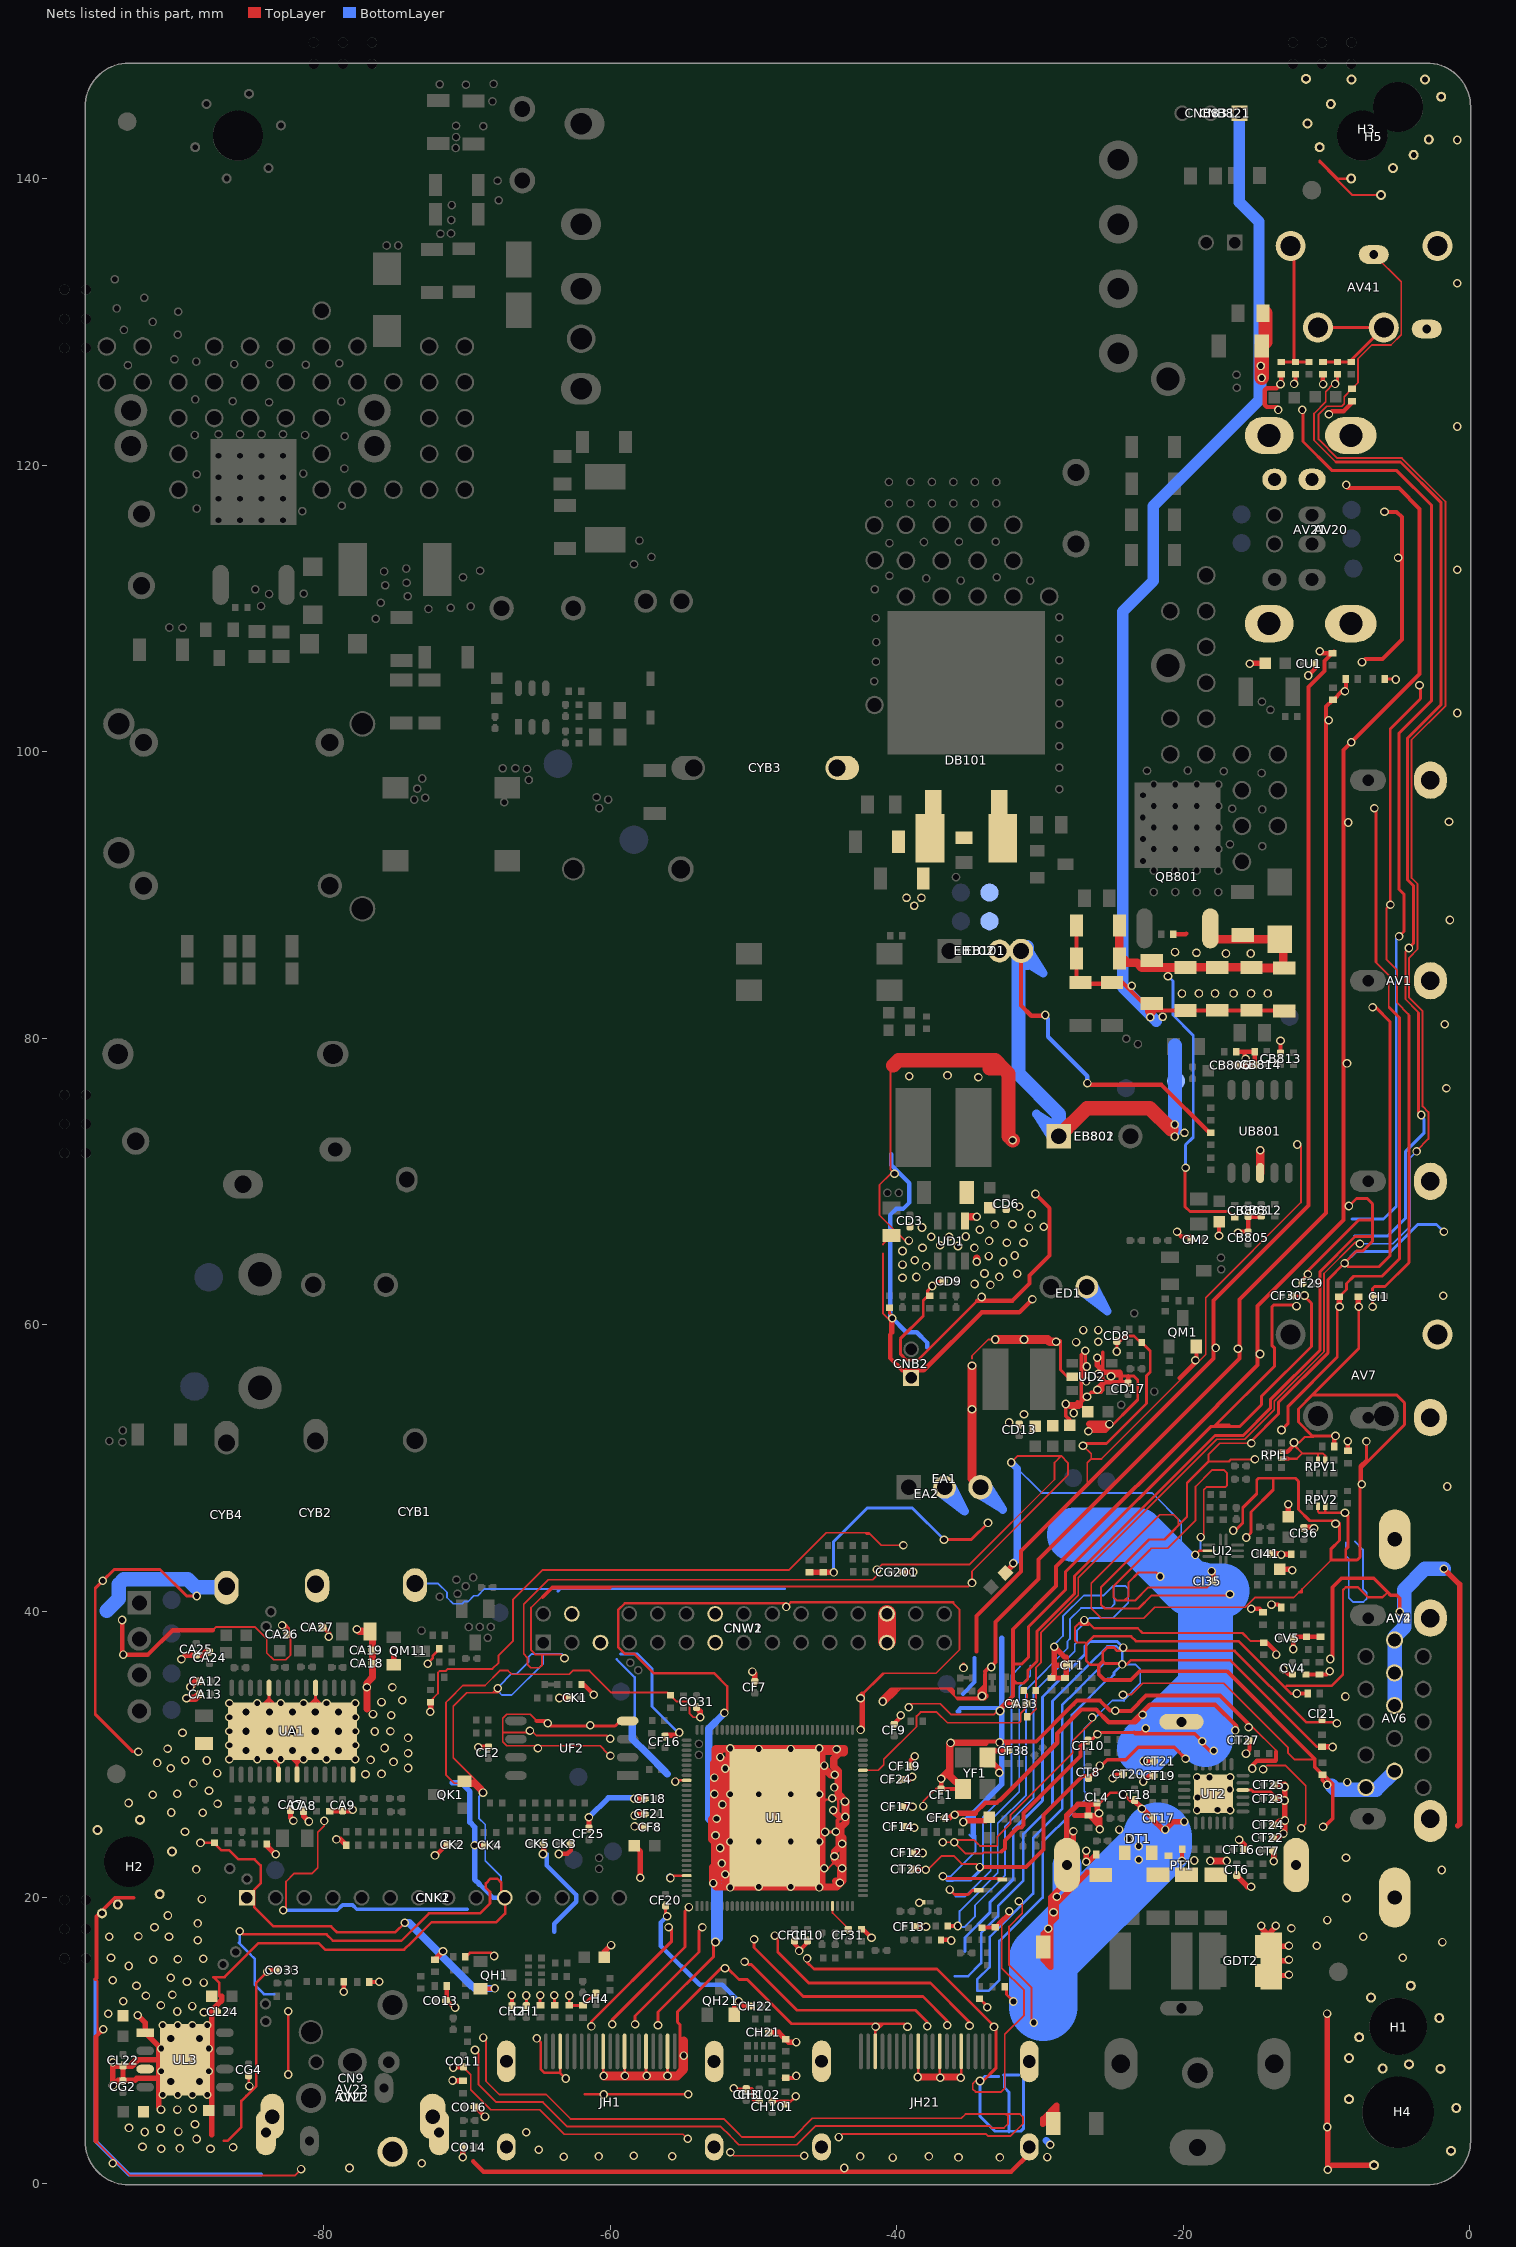
[diagram p0: the nets of this part, all layers, seen from the top]
# Altium PCB MISC86372.PcbDoc (part 8 of 16)
Units mm, origin at the board's own origin, x right, y up, seen from the top; angles counter-clockwise.
Board outline 96.73 x 148.13 mm, 2 copper layers (TopLayer, BottomLayer), stack 1.571 mm thick; 578 components, 318 nets, 2702 pads, 836 vias.

## Via types
v1: diameter 0.6, hole 0.4, TopLayer to BottomLayer, tented both sides, 816 vias
v2: diameter 0.7, hole 0.5, TopLayer to BottomLayer, tented both sides, 15 vias
v3: diameter 0.8, hole 0.5, TopLayer to BottomLayer, tented both sides, 5 vias

## Nets (pads, with @x,y where several pads share a name; then routed paths per layer and width w, separated by ;. In a path a pad name is that pad's centre, name@x,y a point inside that pad or via, vN(x,y) a via of type N, cw(c..) or ccw(c..) an arc to the next point about the centre after c; other vN are vias at no path point) (continued)
EPH_DET_IN: AV41.6 DA33.K RA35.1 RA36.2 | length 129.3
  TopLayer w0.127: RA35.1@-30.792,32.639 -30.284,33.148 RA36.2@-30.284,34.442 -30.284,36.042 -29.939,36.386 -29.939,38.482 -27.33,41.09 -27.33,42.335 -17.671,51.994 -15.703,51.994 -13.652,54.044 -13.652,54.636 ; -13.65,54.635 -10.173,58.112 -10.173,63.563 -7.991,65.746 -7.773,65.746 v1(-7.666,65.638) ; AV41.6@-6.7,134.7 -4.785,132.785 -4.785,129.097 -5.497,128.385 -6.838,128.385 -7.798,127.425 -7.798,125.751 DA33.K@-8.23,125.319 -8.766,124.783 -8.766,124.286 -8.939,124.112 -9.993,124.112 -10.554,123.551 -10.554,121.793 -9.245,120.485 -4.73,120.485 -1.702,117.456 -1.702,103.175 -4.065,100.812 -4.065,91.183 -3.645,90.763 -3.645,86.195 -4.229,85.611 -4.229,82.809 -3.289,81.869 -3.289,75.23 -2.888,74.828 -2.888,72.957 -3.708,72.136 v1(-3.708,72.085)
  BottomLayer w0.127: v1(-7.666,65.638) -5.38,65.638 -4.178,66.84 -4.178,71.615 v1(-3.708,72.085)
EPH_DET_IN_IC: CA33.2@-30.898,33.528 CA33.2@-31.073,33.528 RA36.1 U1.58 | length 16
  TopLayer w0.127: U1.58@-42.363,28.881 -41.3,28.881 -40.907,29.273 -40.907,29.646 -38.617,31.936 -38.617,32.663 -38.337,32.943 -37.204,32.943 -36.459,32.199 -31.45,32.199 -31.344,32.305 -31.344,32.872 -31.073,33.143 CA33.2@-31.073,33.528 ; RA36.1@-31.134,34.442 -30.898,34.206 CA33.2@-30.898,33.528
EPH_LOUT: AV41.4 AV41.5 DA31.K RA31.2 RA34.2 | length 9.8
  TopLayer w0.203: AV41.5@-10.6,129.6 -6.512,129.6 AV41.4@-6.256,129.344 ; DA31.K@-10.251,127.196 RA34.2@-8.27,127.196 -8.27,127.33 AV41.4@-6.256,129.344 ; AV41.4@-6,129.6 AV41.4@-6.256,129.344
EPH_ROUT: AV41.3 DA32.K RA32.2 RA33.2 | length 10.1
  TopLayer w0.203: DA32.K@-13.157,127.196 RA33.2@-11.227,127.196 ; AV41.3@-12.5,135.3 -12.268,135.068 RA32.2@-12.268,127.222
FB: CB129.2 pad.VIA5@-15.291,85.903 pad.VIA5@-17.018,85.903 pad.VIA5@-19.075,85.954 pad.VIA5@-20.574,86.004 QB801.S RB806.1 RB808.2 RB818.1 RB819.1 RB820.1 RB821.1 RB822.1 RB823.1 RB824.1 ZDB801.A | length 45.1
  TopLayer w0.2: v1@-19.866,70.942 -19.866,68.224 -19.533,67.891 -16.859,67.891 -16.462,67.495 RB806.1@-16.408,67.495
  TopLayer w0.3: RB808.2@-20.682,87.249 -19.837,87.249 -19.787,87.3
  TopLayer w0.6: RB822.1@-24.459,87.859 -24.459,85.8 -23.914,85.255 -23.231,85.255 -22.89,84.914 RB824.1@-20.041,84.914 ; -22.291,84.918 -22.271,84.939 RB819.1@-17.628,84.939 -15.342,84.939 -15.291,84.888 -13.03,84.888 ZDB801.A@-13.03,86.671 ; QB801.S@-18.39,87.655 -17.634,86.9 ZDB801.A@-13.259,86.9
  BottomLayer w0.2: v1(-21.065,84.315) -20.726,83.977 -20.726,81.61 -19.306,80.189 -19.306,73.077 -19.837,72.545 v1(-19.837,70.942)
GIN1N: CF31.1 U1.28 | length 1.8
  TopLayer w0.127: U1.28@-44.488,19.406 -44.488,18.929 CF31.1@-43.543,17.983
GND: AV1.2 AV1.4 AV1.6 AV2.2 AV2.4 AV2.6 AV4.2 AV4.4 AV4.6 AV6.5 AV6.6 AV6.7 AV6.8 AV6.10 AV6.16 AV6.17 AV7.1 AV20.4 AV20.5 AV20.6 AV21.4 AV21.8 AV21.9 AV21.10 AV21.11 AV21.12 AV22.2@-71.95,3.6 AV22.3@-84.05,3.6 AV23.4 AV23.5 AV41.1 AV41.2 CA1.1 CA2.1 CA7.1 CA8.1 CA9.1 CA12.1 CA13.1 CA18.1 CA19.1 CA24.1 CA25.2@-88.9,36.913 CA25.2@-88.9,37.088 CA26.1 CA27.2@-80.038,38.869 CA27.2@-80.213,38.869 CA33.1 CB801.2 CB803.2@-15.469,67.52 CB803.2@-15.469,67.695 CB805.1 CB806.2@-16.288,78.105 CB806.2@-16.463,78.105 CB808.1 CB812.1 CB813.1 CB814.2@-14.83,78.13 CB814.2@-15.005,78.13 CD1.1 CD2.2 CD3.1 CD6.1 CD7.1 CD8.1 CD9.1 CD10.1 CD13.1 CD14.1 CD15.1 CD16.1 CD17.1 CD101.A CD102.A CF1.1 CF2.1 CF3.1 CF4.1 CF5.1 CF7.1 CF8.1 CF9.1 CF10.1 CF11.2@-47.14,16.95 CF11.2@-47.14,17.125 CF12.1 CF13.1 CF14.1 CF15.1 CF16.1 CF17.1 CF18.2@-57.459,26.898 CF18.2@-57.634,26.898 CF19.2@-39.021,29.159 CF19.2@-39.196,29.159 CF20.1 CF21.2@-57.451,25.832 CF21.2@-57.626,25.832 CF24.2@-39.78,28.245 CF24.2@-39.605,28.245 CF25.2@-61.493,24.86 CF25.2@-61.493,24.685 CF29.2@-11.553,62.865 CF29.2@-11.728,62.865 CF30.2@-12.344,62.001 CF30.2@-12.519,62.001 CF38.1 CG1.1 CG2.1 CG3.1 CG4.2@-85.25,7.534 CG4.2@-85.25,7.709 CG201.2@-39.58,42.723 CG201.2@-39.755,42.723 CH1.2@-65.862,12.294 CH1.2@-65.862,12.469 CH2.2@-66.861,12.299 CH2.2@-66.861,12.474 CH3.1 CH4.1 CH21.2@-48.888,10.59 CH21.2@-49.063,10.59 CH22.2@-50.078,12.421 CH22.2@-50.253,12.421 CH101.1 CH102.1 CI1.2@-6.6,61.951 CI1.2@-6.775,61.951 CI9.1 CI21.2@-10.312,32.392 CI21.2@-10.312,32.567 CI35.2@-17.91,42.088 CI35.2@-18.085,42.088 CI36.1 CI40.1 CI41.1 CK1.1 CK2.1 CK3.1 CK4.2@-68.62,23.63 CK4.2@-68.795,23.63 CK5.2@-64.631,23.752 CK5.2@-64.806,23.752 CL3.1 CL4.1 CL21.2 CL22.2@-94.018,8.39 CL22.2@-94.018,8.215 CL23.2 CL24.1 CM2.1 CN1.2@-71.95,3.6 CN1.3@-84.05,3.6 CN9.1 CNB2.1 CNB821.1 CNB831.1 CNK1.1 CNK1.10 CNK2.1 CNK2.10 CNW1.4 CNW1.5 CNW1.13 CNW1.14 CNW1.25 CNW1.26 CNW2.4 CNW2.5 CNW2.13 CNW2.14 CNW2.25 CNW2.26 CO11.1 CO13.1 CO14.1 CO16.1 CO31.1 CO33.1 CT1.2@-27.987,36.22 CT1.2@-28.162,36.22 CT6.1 CT7.1 CT8.1 CT10.2@-26.645,30.832 CT10.2@-26.645,31.007 CT16.2@-15.704,23.343 CT16.2@-15.879,23.343 CT17.1 CT18.2@-23.393,26.753 CT18.2@-23.393,26.928 CT19.1 CT20.2@-24.079,28.6 CT20.2@-24.254,28.6 CT21.1 CT22.2@-13.692,24.154 CT22.2@-13.867,24.154 CT23.1 CT24.1 CT25.2@-13.596,27.864 CT25.2@-13.771,27.864 CT26.1 CT27.1 CT41.1 CT42.1 CT43.1 CT44.1 CT45.1 CT46.1 CT47.1 CT48.1 CU1.2@-10.772,106.147 CU1.2@-10.947,106.147 CU2.2 CV4.1 CV5.1 CYB1.2 CYB2.2 CYB3.2 CYB4.2 DA31.A DA32.A DA33.A DB101.1 DB101.3 DH1.A DH2.A DH3.A DH21.A DH22.A DH23.A DH81.A DI1.A DI2.A DI3.A DI6.A DI8.A DI9.A DK1.A DK2.A DK3.A DO1.A DT1.1 DT1.3 DU1.A DU2.A DU3.A DU4.A DV1.A DV2.A DV3.A DV4.A DV5.A DV6.A DV7.A DV8.A DV9.A EA1.2 EA2.2 EB101.2 EB102.2 EB801.1@-28.687,73.139 EB802.1 ED1.2 GDT2.2@-13.851,15.57 GDT2.2@-14.501,14.554 GDT2.2@-14.501,16.586 H1.1 H1.2 H1.3 H1.4 H1.5 H1.6 H2.1 H2.2 H2.3 H2.4 H2.5 H2.6 H3.1 H3.2 H3.3 H3.4 H3.5 H3.6 H4.1 H4.2 H4.3 H4.4 H4.5 H4.6 H5.1 H5.2 H5.3 H5.4 H5.5 H5.6 JH1.2 JH1.5 JH1.8 JH1.11 JH1.17 JH1.20 JH1.21 JH1.22 JH1.23 JH21.5 JH21.8 JH21.11 JH21.17 JH21.20 JH21.21 JH21.22 JH21.23 LF6.JP_2K LT2.2 LT3.2 LT4.2 LT5.2 pad.VIA5@-14.58,126.924 pad.VIA5@-14.097,83.114 pad.VIA5@-14.527,126.087 pad.VIA5@-15.265,83.114 pad.VIA5@-16.485,83.114 pad.VIA5@-17.78,83.114 pad.VIA5@-18.907,83.114 pad.VIA5@-19.914,73.381 pad.VIA5@-20.091,83.109 pad.VIA5@-20.599,73.127 pad.VIA5@-20.599,73.965 pad.VIA5@-21.438,81.483 pad.VIA5@-22.301,81.458 pad.VIA5@-23.597,83.642 pad.VIA5@-38.278,89.789 pad.VIA5@-38.786,89.23 pad.VIA5@-39.319,89.789 PT1.2 PT1.3 PT1.4 QH1.E QH21.E QK1.E QM1.E QM11.E RA1.2 RA4.JP_2K RA5.JP_2K RA9.1 RA11.1 RA31.1 RA32.1 RB128.2 RB129.2 RB134.1 RB140.2 RB803.1 RB818.2 RB819.2 RB820.2 RB821.2 RB822.2 RB823.2 RB824.2 RB825.1 RB826.1 RB833.1 RB847.1 RD5.1 RD6.1 RD8.2 RF12.2 RF13.2 RF16.2 RH82.2 RI1.1 RI43.1 RM12.2 RM15.2 RO1.1 RO4.1 RO22.1 RPI1.3 RPI1.5 RPV1.3 RPV1.5 RPV2.3 RPV2.5 RV1.1 RV3.1 RV5.1 RV6.1 RV8.1 TP_12VA-.1 TP_12VB-.1 TP_LED+.1 U1.105 U1.124 U1.EPAD UA1.6 UA1.8 UA1.14 UA1.19 UA1.24 UA1.EPAD@-82.197,31.611 UB801.3 UD1.1 UD2.2 UF2.4 UI2.4 UL3.1 UL3.3 UL3.EPAD UT2.10 UT2.25 YF1.2 YF1.4 | length 3376.3
  TopLayer w0.127: -95.94,14.301 -95.796,14.157 -95.796,2.856 -93.535,0.596 -93.417,0.596 -93.406,0.584 -82.042,0.584 v1(-81.585,1.041) ; -87.757,38.648 -87.517,38.887 -84.808,38.887 -83.979,38.058 -83.979,37.071 -83.509,36.601 -82.648,36.601 -82.321,36.928 -82.321,38.191 CA26.1@-82.502,38.372 ; v1(-82.912,39.01) v1@-82.778,39.01 ; v1(-82.828,19.109) -82.796,19.109 v1@-82.639,19.266 ; v1@-82.639,19.201 v1@-82.639,19.266 ; -82.639,19.563 v1@-82.639,19.266 ; v1(-79.973,25.346) -79.973,25.011 -80.416,24.568 -80.416,22.065 -80.802,21.68 -82.072,21.68 -82.639,21.113 v1@-82.639,19.266 ; RM12.2@-72.542,33.636 -72.542,33.73 -72.026,34.247 -72.026,35.705 -71.923,35.808 -71.499,35.808 -71.347,35.96 ; RM12.2@-72.441,33.636 RM12.2@-72.441,33.777 ; -71.476,28.56 -70.893,27.978 QK1.E@-70.053,27.978 ; -71.476,28.576 -71.476,33.611 -71.249,33.838 -70.289,34.798 -68.747,34.798 -67.705,35.839 -67.142,35.839 -66.888,35.585 -62.861,35.585 -62.607,35.839 -61.461,35.839 -59.928,34.306 -56.004,34.306 RO22.1@-55.804,34.105 -55.372,33.674 -54.596,33.674 -54.465,33.542 -54.465,32.829 -54.214,32.578 v1(-53.722,32.578) ; -71.476,35.831 -71.347,35.96 ; CO11.1@-70.256,8.135 -69.742,7.62 -69.742,6.572 -68.351,5.182 -64.925,5.182 -63.219,3.476 -54.924,3.476 v1(-54.597,3.15) ; v1(-69.445,9.356) -69.208,9.119 -69.208,8.28 ; -69.208,9.061 -69.208,8.28 ; QH1.E@-69.063,13.361 QH1.E@-69.063,13.627 ; v1@-68.883,27.388 -68.883,27.658 -70.968,29.743 -70.968,33.347 -70.024,34.29 -68.809,34.29 ; v1(-68.874,10.221) -68.675,10.022 -68.675,8.941 ; v1@-68.864,10.447 -68.675,10.257 -68.675,8.941 ; -68.675,9.296 -68.675,8.941 ; v1(-67.849,34.607) -67.908,34.607 -68.224,34.29 -68.809,34.29 ; v1@-67.809,34.382 v1@-67.766,34.339 ; v1@-67.784,34.357 -67.851,34.29 -68.809,34.29 ; -67.502,31.52 -65.367,31.52 -65.156,31.309 -64.77,31.309 ; -65.134,32.325 -65.134,32.339 -65.587,32.791 -67.228,32.791 -67.502,32.517 -67.502,30.862 -67.23,30.59 -66.675,30.59 v1@-65.07,30.59 ; v1(-65.049,30.42) -65.07,30.44 v1@-65.07,30.59 ; -64.926,31.309 -64.77,31.309 ; -64.77,36.973 -64.762,36.965 -64.762,36.228 -64.948,36.043 -65.557,36.043 -65.787,36.272 -65.787,36.751 -66.04,37.004 -66.04,40.485 -64.336,42.189 -41.682,42.189 -41.377,42.494 v1(-41.377,42.891) -41.012,43.256 -34.916,43.256 -28.989,49.182 -28.989,50.363 -28.527,50.825 ; v1(-63.195,36.703) -63.465,36.973 -65.25,36.973 -65.532,37.255 -65.532,40.247 -64.056,41.723 -34.985,41.723 v1(-34.747,41.961) -34.747,42.778 -28.05,49.475 -28.05,50.348 -28.527,50.825 ; v1@-60.5,7.592 v1(-60.452,7.544) ; v1(-59.995,31.09) -60.214,31.309 -64.77,31.309 ; v1(-59.99,29.888) -59.99,30.075 -60.197,30.075 -60.712,30.59 v1@-65.07,30.59 ; v1@-59,7.565 v1(-58.979,7.544) ; v1@-57.5,7.589 v1(-57.455,7.544) ; v1(-51.613,2.21) -51.37,1.967 v1(-46.457,1.967) ; CH101.1@-48.819,5.81 -48.157,5.81 -48.142,5.795 DH21.A@-47.904,5.557 ; v1(-44.043,3.277) -43.822,3.497 -33.788,3.497 -33.647,3.356 -32.041,3.356 -31.176,4.221 -31.176,4.66 -31.394,4.879 -32.385,4.879 ; v1(-42.534,33.916) -42.534,33.997 -40.871,35.661 -39.751,35.661 ; v1(-42.524,31.699) -42.524,34.133 -40.996,35.661 -39.751,35.661 ; -42.193,45.469 -42.088,45.364 -41.859,45.364 -41.656,45.161 ; -40.97,64.957 -40.97,60.778 -40.464,60.272 -40.464,59.297 ; -40.97,65.593 CD2.2@-40.361,66.202 ; -40.299,33.999 -39.704,34.594 -39.319,34.594 ; -40.244,78.078 -40.437,77.886 -40.437,70.815 v1(-40.157,70.536) -40.424,70.536 -41.206,69.755 -41.206,67.638 v1@-39.16,65.593 ; v1(-39.533,44.593) -41.088,44.593 -41.656,45.161 ; v1@-39.262,33.527 -38.913,33.527 ; v1(-39.167,33.274) -38.913,33.527 ; v1(-38.424,19.639) LF6.JP_2K@-38.276,19.787 ; v1(-38.145,26.381) -38.145,26.716 -37.764,27.096 ; -38.1,26.761 -37.764,27.096 ; v1@-38.001,21.971 -37.795,21.971 -36.865,22.901 -36.036,22.901 -35.478,22.342 -34.434,22.342 v1(-34.215,22.123) ; CF1.1@-36.906,27.603 -37.258,27.603 -37.764,27.096 ; v1(-36.782,23.858) -35.992,23.858 v1(-35.987,23.863) -35.84,24.011 -34.603,24.011 -34.341,23.749 ; -36.068,40.538 -35.611,40.081 -35.611,37.313 -37.262,35.661 -39.751,35.661 ; v1@-35.983,23.867 -35.179,23.063 -34.012,23.063 -33.936,23.139 -32.856,23.139 -32.512,23.483 -32.512,24.027 -31.645,24.894 -31.294,24.894 ; -35.806,33.934 -35.844,33.972 -35.878,33.972 -35.989,34.084 ; -34.748,57.619 -34.748,57.823 -33.618,58.953 v1(-33.122,58.953) ; -34.526,23.935 -34.341,23.749 ; v1(-34.188,7.188) -34.514,7.188 -34.69,7.012 -34.69,6.625 -34.493,6.428 -32.708,6.428 -32.457,6.68 -32.457,10.448 -31.112,11.793 -31.112,13.514 -32.664,15.067 -32.664,18.194 ; -33.733,34.133 -33.733,34.052 ; -33.717,34.036 -33.733,34.052 ; v1@-33.467,36.027 -33.776,35.719 ; v1(-33.401,36.092) -33.403,36.092 -33.776,35.719 ; v1@-32.756,33.229 -33.219,32.766 -36.2,32.766 -36.962,33.527 -38.913,33.527 ; -32.664,18.371 -32.664,18.194 ; v1@-32.136,18.801 -32.156,18.821 -32.156,18.702 -32.664,18.194 ; v1(-32.007,50.368) -31.549,50.825 -28.527,50.825 ; v1(-31.471,19.736) -31.234,19.499 -31.234,18.899 -32.156,17.977 -32.156,15.277 -30.604,13.724 -30.604,11.443 v1(-30.429,11.269) ; -27.331,48.183 -26.703,48.81 -26.703,50.347 -26.428,50.622 ; v1(-27,51.537) -26.428,50.965 -26.428,50.622 ; -26.55,32.106 -26.762,31.893 ; v1(-26.365,32.571) -26.365,32.29 -26.762,31.893 ; -24.735,32.326 -23.226,32.326 ; v1@-24.206,34.328 v1(-24.206,34.163) -23.622,34.163 -22.824,34.96 -17.18,34.96 -12.695,30.475 -12.695,30.094 -12.243,29.642 -10.82,29.642 ; -23.558,32.237 -23.315,32.237 ; -22.345,44.256 -22.222,44.38 -21.084,44.38 -19.139,46.325 -19.139,48.694 -17.999,49.834 -17.144,49.834 -16.942,49.632 -16.942,48.793 -17.081,48.654 -18.377,48.654 -18.567,48.463 -18.567,45.364 v1(-18.771,45.161) ; -20.395,45.913 -20.354,45.954 -20.354,46.422 -20.651,46.718 -21.629,46.718 -26.416,41.932 -26.416,40.183 -25.732,39.498 -22.757,39.498 -21.996,40.259 -15.672,40.259 -14.993,40.938 -12.301,40.938 -11.709,41.529 ; CT43.1@-19.788,21.591 CT43.1@-19.406,21.974 ; -18.233,50.444 -18.233,50.93 -17.448,51.714 v1(-15.24,51.714) ; v1@-15.628,30.055 v1@-15.579,30.055 ; v1(-15.439,31.885) -15.137,31.885 -13.523,30.271 -13.523,30.177 ; v1(-15.189,29.007) v1@-15.164,28.981 ; v1(-14.427,28.956) v1@-14.415,28.944 ; -14.173,29.21 -12.849,29.21 -11.453,27.813 -11.453,26.479 -11.448,26.474 -11.448,25.154 v1(-11.76,24.841) ; v1(-12.04,72.568) -11.913,72.568 -11.786,72.441 -11.786,68.521 -18.422,61.884 -18.422,57.908 -25.708,50.622 -26.428,50.622 ; -11.915,41.324 -11.87,41.279 -11.72,41.279 ; -11.871,41.368 -11.809,41.368 -11.72,41.279 ; v1@-10.472,25.034 -10.328,25.034 v1(-10.236,24.942) ; -9.874,63.151 v1(-8.738,64.287) ; -9.685,43.553 -11.709,41.529 ; v1(-9.402,125.669) -9.521,125.669 -10.056,125.134 -10.056,124.408 -10.871,123.593 -10.871,121.742 -9.347,120.218 ; -6.54,85.324 -6.54,85.271 -5.651,84.382 -5.651,82.166 -5.613,82.128 ; v1@-5.551,89.32 -5.799,89.072 -5.799,85.463 -5.067,84.731 -5.067,82.462 -4.28,81.675 ; v1(-4.247,86.287) -4.483,86.05 -4.483,82.704 -3.619,81.84 ; -71.347,35.96 -68.231,35.96 -67.793,36.399 -67.793,36.912 -66.802,37.902 -66.802,38.429 -66.802,40.801 -64.728,42.875 -47.519,42.875 -44.925,45.469 -41.964,45.469 -41.656,45.161 ; -69.208,8.28 -69.208,6.954 -67.969,5.715 -64.704,5.715 -62.999,4.01 -52.286,4.01 -51.63,3.354 -51.63,3.35 -51.024,2.743 -46.981,2.743 -45.668,4.056 -33.521,4.056 -33.38,3.915 -32.511,3.915 -32.225,4.202 -32.225,4.719 -32.385,4.879 ; -68.675,8.941 -68.675,7.175 -67.748,6.248 -64.483,6.248 -62.778,4.543 -52.065,4.543 -51.097,3.575 -51.097,3.571 -50.803,3.277 -47.202,3.277 -45.889,4.589 -35.49,4.589 -35.201,4.879 -32.385,4.879 ; -39.726,34.594 -40.056,34.594 v1(-40.97,33.68) -40.792,33.68 -39.879,34.594 -39.726,34.594 ; -39.726,34.594 -39.319,34.594 ; -39.319,34.594 -36.52,34.594 ; -36.52,34.594 -35.758,33.833 -34.56,33.833 ; -36.52,34.594 -36.323,34.594 ; -36.323,34.594 -35.989,34.261 ; -36.323,34.594 -36.16,34.594 -35.989,34.424 -35.989,34.261 ; -36.323,34.594 -36.323,34.418 -35.989,34.084 ; -35.989,34.084 -35.989,34.261 ; -34.56,33.833 -34.521,33.871 -34.458,33.934 -34.27,34.122 -33.927,34.466 -33.902,34.49 ; -34.56,33.833 -33.822,33.833 -33.665,33.99 -33.665,34.149 -33.776,34.261 -33.776,34.34 ; -34.341,23.749 -34.188,23.597 -33.045,23.597 -32.985,23.657 -32.985,24.24 -32.052,25.172 -32.052,25.763 -27.713,30.102 -27.713,30.942 -26.762,31.893 ; v1@-33.902,34.214 -33.902,34.466 ; v1@-33.902,34.214 v1(-34.046,34.069) -33.75,34.069 -33.733,34.052 ; v1@-33.902,34.214 -33.776,34.34 ; -33.902,34.466 -33.776,34.34 ; -33.902,34.466 -33.902,34.49 ; -33.902,34.49 -33.902,34.776 -33.902,35.593 -33.776,35.719 ; -33.776,34.34 -33.776,35.719 ; -11.72,41.279 -11.709,41.289 -11.709,41.529
  TopLayer w0.152: v1(-55.474,28.092) -55.385,28.181 U1.105@-54.664,28.181 ; v1@-55.372,28.296 -55.474,28.296 v1@-55.359,28.181 ; v1@-52.553,24.511 -52.578,24.536 v1(-52.578,25.502) -52.524,25.556 -51.713,25.556 U1.EPAD@-50.863,25.556 ; v1@-52.451,27.178 -52.451,29.337 ; -52.375,21.298 -51.713,21.96 -48.513,25.16 U1.EPAD@-48.513,25.556 ; -52.307,20.735 -48.513,24.529 U1.EPAD@-48.513,25.556 ; v1@-52.222,22.21 -51.713,22.719 U1.EPAD@-48.877,25.556 ; v1(-51.97,21.62) -52.192,21.62 v1(-52.807,21.006) -52.807,21.047 -52.473,21.381 -52.172,21.682 -48.513,25.341 U1.EPAD@-48.513,25.556 ; v1(-51.968,29.007) -51.968,29.451 v1(-52.322,29.805) -48.513,25.996 U1.EPAD@-48.513,25.556 ; -51.713,26.406 U1.EPAD@-50.863,25.556 ; v1(-45.06,22.047) -44.78,22.047 -44.247,22.581 ; v1@-45.06,24.536 v1@-44.806,24.536 ; -45.06,26.695 -44.905,26.85 -44.138,26.85 ; v1@-45.009,24.333 v1@-44.806,24.536 ; v1(-45.004,24.57) -44.988,24.587 v1@-44.755,24.587 ; v1(-44.37,27.686) -44.138,27.455 ; -44.194,23.647 v1@-44.194,24.64 ; v1@-44.176,30.381 -44.323,30.234 -44.323,29.767 -44.323,29.06 v1(-44.323,28.575) -44.138,28.39 -44.138,27.455 ; -26.774,37.716 -26.853,37.795 -27.416,37.795 -27.554,37.933 -27.554,38.867 -27.056,39.365 -26.792,39.365 -26.627,39.2 ; v1(-22.768,29.531) v1@-22.753,29.515 ; -22.345,44.256 -24.862,41.74 -24.862,40.958 -24.632,40.729 -24.105,40.729 ; -21.896,42.683 -22.276,42.683 ; v1(-21.6,42.408) -21.875,42.683 -22.276,42.683 ; v1(-18.023,42.79) v1@-17.91,42.677 ; CI35.2@-17.91,42.088 -18.346,41.651 -22.433,41.651 -23.355,40.729 -24.105,40.729 ; v1(-16.739,41.173) -16.82,41.092 -22.202,41.092 -23.124,40.17 -25.463,40.17 -25.751,40.457 -25.751,41.641 -22.393,44.999 -21.31,44.999 -19.736,46.573 -19.736,48.941 -18.233,50.444 -16.81,50.444 -16.675,50.579 -15.002,50.579 v1(-14.994,50.587) ; CT27.1@-15.272,30.836 CT27.1@-15.272,31.032 ; DI1.A@-14.314,37.751 -14.363,37.8 -14.46,37.897 -15.291,37.897 -15.862,38.468 -22.847,38.468 -23.179,38.8 -26.227,38.8 -26.627,39.2 ; -12.7,50.626 -12.07,50.626 -11.688,51.008 ; v1@-12.268,51.587 -11.688,51.008 ; v1(-12.268,51.765) -11.896,51.765 -11.508,52.153 -10.926,52.153 ; -10.617,51.008 -10.592,50.982 RPV1.5@-10.592,50.532 ; RPV2.3@-10.592,47.309 -10.592,46.939 -10.516,46.863 -8.718,46.863 v1(-8.707,46.853) ; -10.109,46.863 -10.092,46.88 RPV2.5@-10.092,47.309 ; RPV1.3@-10.092,50.532 -10.092,50.841 -10.258,51.008 -11.688,51.008 ; -8.85,35.575 -8.85,41.467 -8.661,41.656 -7.798,41.656 -7.099,40.957 -6.083,40.957 -5.728,41.313 ; H3.1@-8.278,140.006 -9.343,140.006 ; H3.1@-8.23,139.979 -9.197,139.979 -10.479,141.262 -10.479,141.142 -9.343,140.006 ; H5.1@-6.198,138.862 -8.199,138.862 -9.343,140.006 ; U1.EPAD@-50.863,25.556 U1.EPAD@-48.877,25.556 ; U1.EPAD@-48.877,25.556 U1.EPAD@-48.513,25.556 ; v1@-44.806,24.536 v1@-44.755,24.587 ; v1@-44.806,24.536 -44.298,24.536 v1(-44.247,24.587) ; v1@-44.755,24.587 v1(-44.247,24.587) ; v1(-44.247,24.587) v1@-44.194,24.64 ; v1@-44.194,24.64 -44.091,24.743 -44.091,25.522 ; v1@-44.194,24.64 -44.194,25.418 -44.091,25.522 ; -44.138,26.85 -44.138,27.455 ; -44.138,26.85 -44.091,26.802 -44.091,25.522 ; -26.627,39.2 -26.627,39.048 -26.619,39.04 -27.158,39.04 -27.27,39.151 -26.676,39.151 -26.627,39.2 ; -24.105,40.729 -23.813,41.021 -23.813,41.999 -23.129,42.683 -22.276,42.683
  TopLayer w0.178: v1(-88.609,23.811) RA1.2@-87.874,23.811 ; RA1.2@-87.671,23.811 -87.164,23.303 -86.606,23.303 -85.959,22.657 -85.118,22.657 ; -87.289,13.106 -87.289,14.024 -87.704,14.439 -86.924,14.439 -84.548,16.815 -80.366,16.815 -79.908,16.358 -74.386,16.358 -73.891,16.853 ; -86.995,3.015 -86.713,3.015 -85.75,3.978 -85.75,5.798 -85.411,6.137 -85.411,6.142 -84.709,6.844 -84.709,14.056 v1(-83.957,14.808) ; v1(-85.87,17.644) -85.65,17.424 -79.807,17.424 -79.362,16.98 -74.586,16.98 -72.668,18.898 -70.409,18.898 ; -85.408,22.657 -84.828,22.657 -84.417,22.246 -84.417,20.98 -84.861,20.536 -84.861,19.344 -83.5,17.983 -79.493,17.983 ; CG4.2@-85.25,7.709 -85.25,6.891 v1(-85.192,6.833) ; v1(-82.474,7.645) -82.474,11.1 ; -82.474,11.615 -82.474,11.1 ; v1(-82.474,12.065) -82.474,11.1 ; -79.138,17.628 -79.493,17.983 ; v1(-74.346,18.237) -75.019,17.564 -79.074,17.564 -79.493,17.983 ; -73.889,16.853 -73.891,16.853 ; v1(-72.746,36.322) -72.746,36.359 -72.385,36.719 -72.385,36.886 -71.926,37.345 RM15.2@-71.926,37.363 ; CO13.1@-71.406,12.802 -71.313,12.802 v1(-70.835,12.324) ; RH82.2@-70.111,15.811 -69.792,16.129 -68.321,16.129 v1(-68.11,15.918) ; -69.698,18.898 -70.409,18.898 ; CNK2.10@-67.621,19.99 CNK2.10@-67.365,19.99 CNK2.10@-67.347,19.972 ; v1(-65.126,10.16) -64.846,9.881 -64.846,7.994 -64.608,7.756 -63.5,7.756 ; JH1.17@-63.5,9.258 -63.5,7.756 ; v1(-63.11,7.366) -63.5,7.756 ; -61.763,6.274 v1@-60.427,6.274 ; v1@-60.5,7.592 JH1.11@-60.5,9.258 ; v1(-60.452,6.248) v1@-60.427,6.274 ; v1@-59,7.565 JH1.8@-59,9.258 ; v1(-55.804,21.361) -55.635,21.531 U1.124@-54.663,21.531 ; v1(-54.559,6.274) v1@-60.427,6.274 ; v1(-52.03,32.887) -51.841,33.075 -51.841,34.747 -52.756,35.662 -56.978,35.662 -58.347,37.03 -58.999,37.03 -59.447,37.479 -59.447,40.078 -58.988,40.537 -49.416,40.537 ; -49.422,40.53 -49.416,40.537 ; v1(-47.714,40.288) -47.402,40.599 -36.068,40.599 ; v1@-47.714,40.44 -47.714,40.537 -49.416,40.537 ; CL4.1@-26.01,26.563 -25.848,26.563 -25.111,27.301 -24.278,27.301 v1(-24.181,27.203) ; -25.852,36.241 -26.462,36.241 -26.774,36.553 -26.774,37.716 -26.262,38.228 -23.636,38.228 -23.305,37.897 -16.131,37.897 -12.474,34.239 v1(-12.065,34.239) ; v1(-19.156,43.917) -18.864,44.208 UI2.4@-18.206,44.208 ; -12.776,34.798 -9.627,34.798 -8.85,35.575 ; DV5.A@-10.312,30.512 -10.651,30.512 -16.689,36.551 -23.672,36.551 -23.952,36.271 v1(-24.257,36.271) -24.321,36.335 -25.474,36.335 -25.616,36.477 -25.616,37.133 -25.296,37.453 -24.843,37.453 -24.615,37.224 -24.403,37.224 v1(-24.18,37.447) -23.957,37.224 -16.41,37.224 -11.426,32.239 -9.354,32.239 v1(-9.271,32.156) ; -73.891,16.853 -72.465,18.279 -67.945,18.279 -67.347,18.877 CNK2.10@-67.347,19.972 ; -70.409,18.898 -69.086,18.898 -68.395,19.588 -68.395,20.391 -68.682,20.677 -68.682,20.989 -68.347,21.324 -67.89,21.324 -67.623,21.057 -67.623,20.248 CNK2.10@-67.347,19.972